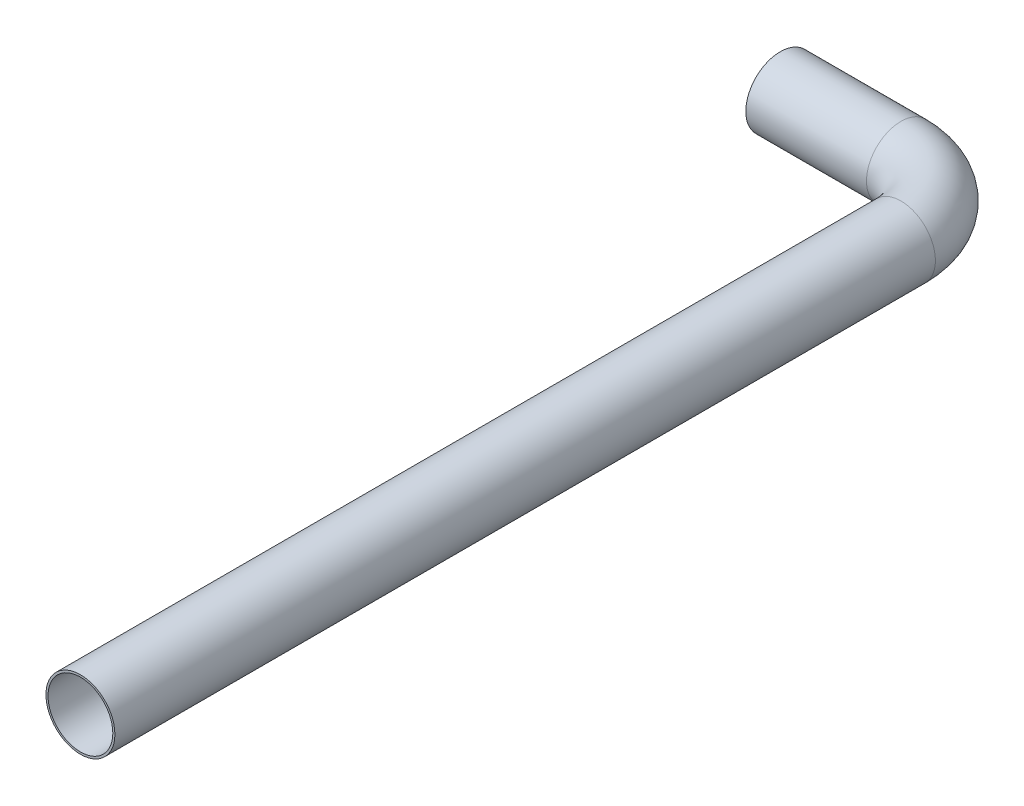
SolidWorks part; units mm, degrees
ref_plane "前视基准面" through (0, 0, 0) normal (0, 0, 1) x (1, 0, 0)
ref_plane "上视基准面" through (0, 0, 0) normal (0, 1, 0) x (1, 0, 0)
ref_plane "右视基准面" through (0, 0, 0) normal (1, 0, 0) x (0, 0, -1)
sketch "草图1" plane through (0, 0, 0) normal (0, 0, 1) x (1, 0, 0)
  circle A0 centre (0, 0) radius 50
  dimension "D1" = 100
sketch "草图2" plane through (0, 0, 0) normal (0, 1, 0) x (1, 0, 0)
  line L0 (0, 0) -> (0, 1190)
  line L1 (-100, 1290) -> (-275, 1290)
  arc A0 (0, 1190) -> (-100, 1290) centre (-100, 1190) ccw
  point P6 (0, 1290)
  dimension "D3" = 100
  dimension "D1" = 1290
  dimension "D2" = 275
sweep "扫描1" add profiles "草图1" path "草图2"
shell "抽壳1" thickness 3
